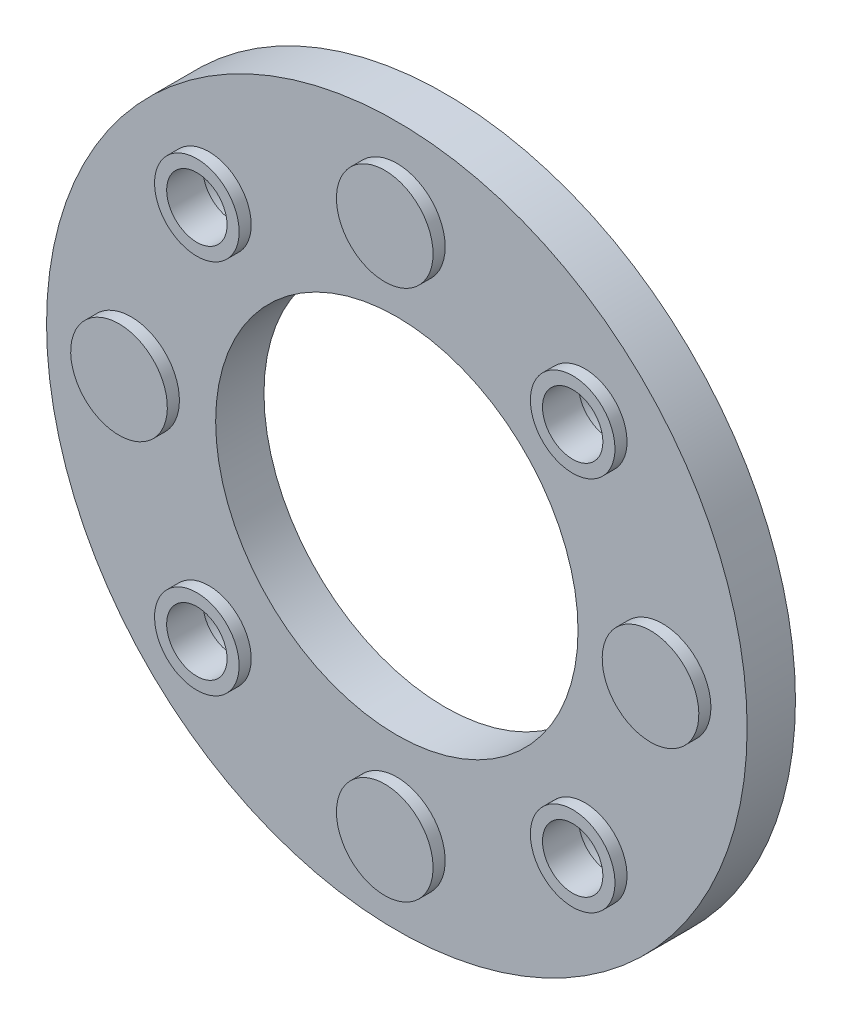
SolidWorks part; units mm, degrees
ref_plane "Front Plane" through (0, 0, 0) normal (0, 0, 1) x (1, 0, 0)
ref_plane "Top Plane" through (0, 0, 0) normal (0, 1, 0) x (1, 0, 0)
ref_plane "Right Plane" through (0, 0, 0) normal (1, 0, 0) x (0, 0, -1)
other "Configuration Table"
sketch "Sketch1" plane through (0, 0, 0) normal (0, 0, 1) x (1, 0, 0)
  circle A0 centre (0, 0) radius 29
  dimension "D1" = 58
extrude "Boss-Extrude1" add sketch "Sketch1" along normal blind 4
sketch "Sketch2" plane through (0, 0, 4) normal (0, 0, 1) x (1, 0, 0)
  circle A0 centre (0, 0) radius 15
  dimension "D1" = 30
extrude "Cut-Extrude1" cut sketch "Sketch2" against normal blind 24
sketch "Sketch3" plane through (0, 0, 4) normal (0, 0, 1) x (1, 0, 0)
  circle A0 centre (0, 22) radius 4
  dimension "D1" = 8
  dimension "D2" = 22
extrude "Boss-Extrude2" add sketch "Sketch3" along normal blind 1
sketch "Sketch5" plane through (0, 0, 0) normal (0, 0, -1) x (-1, 0, 0)
  circle A0 centre (0, 22) radius 2.5
  dimension "D1" = 5
  dimension "D2" = 22
extrude "Cut-Extrude2" cut sketch "Sketch5" against normal blind 4.5
pattern_circular "CirPattern1" count 4 over 360 about axis through (0, 0, 0) along (0, 0, 1) of "Cut-Extrude2", "Boss-Extrude2"
sketch "Sketch6" plane through (0, 0, 4) normal (0, 0, 1) x (1, 0, 0)
  line L0 (0, 0) -> (0, 10.3926)
  line L1 (0, 0) -> (-15.9543, 15.9543)
  circle A1 centre (-15.5563, 15.5563) radius 3.5
  dimension "D2" = 7
  dimension "D1" = 45
  dimension "D3" = 22
extrude "Boss-Extrude3" add sketch "Sketch6" along normal blind 1
sketch "Sketch7" plane through (0, 0, 0) normal (0, 0, -1) x (-1, 0, 0)
  line L0 (0, 0) -> (0, 13.0391)
  line L1 (0, 0) -> (16.5459, 16.5459)
  circle A0 centre (15.5563, 15.5563) radius 3.5
  dimension "D3" = 7
  dimension "D1" = 45
  dimension "D2" = 22
extrude "Cut-Extrude3" cut sketch "Sketch7" against normal blind 2
sketch "Sketch8" plane through (0, 0, 2) normal (0, 0, -1) x (-1, 0, 0)
  circle A1 centre (15.5563, 15.5563) radius 2.5
  dimension "D1" = 5
extrude "Cut-Extrude4" cut sketch "Sketch8" against normal blind 10
pattern_circular "CirPattern2" count 4 over 360 about axis through (0, 0, 0) along (0, 0, 1) of "Boss-Extrude3", "Cut-Extrude3", "Cut-Extrude4"
